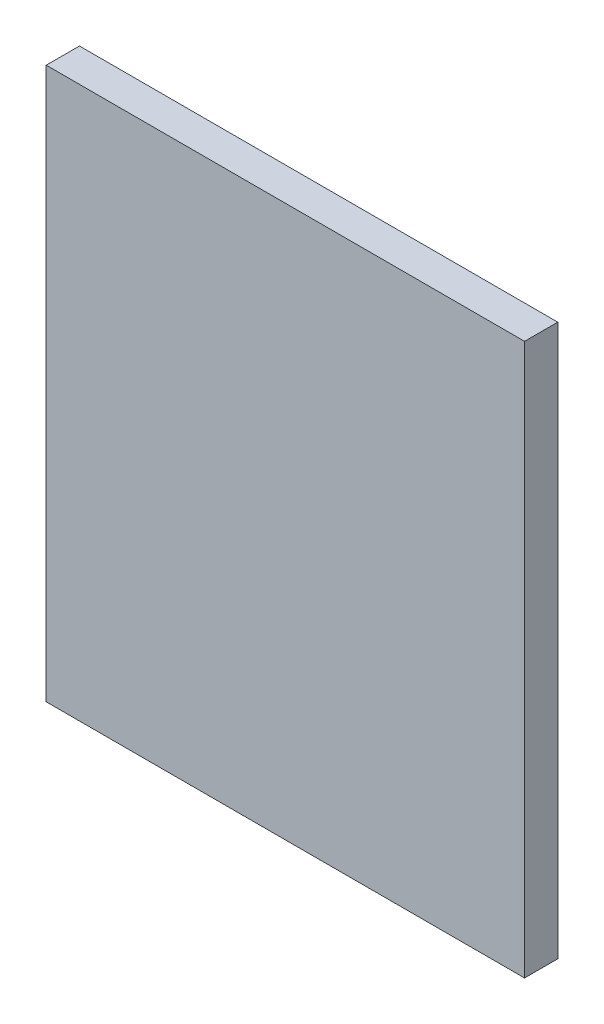
from build123d import *

# Parameters (mm, degrees)
SKETCH1_W           = 360
SKETCH1_H           = 415
BOSS_EXTRUDE1_DEPTH = 25


with BuildPart() as part:
    # Sketch1 → Boss-Extrude1 (new body)
    with BuildSketch(Plane.XY):
        with Locations((180, -207.5)):
            Rectangle(SKETCH1_W, SKETCH1_H)
    extrude(amount=BOSS_EXTRUDE1_DEPTH)


solid = part.part
